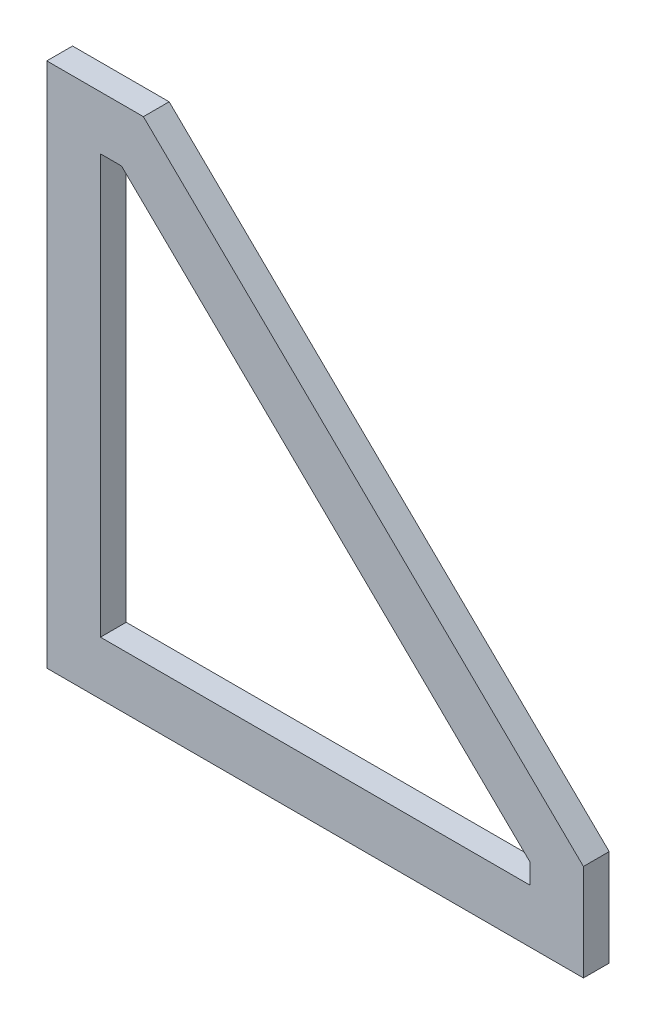
from build123d import *

# Parameters (mm, degrees)
EXTRUDE_1_DEPTH = 6


with BuildPart() as part:
    # 草图1 → 凸台-拉伸1 (new, symmetric)
    with BuildSketch(Plane.XY):
        Polygon((0, 0), (-250, 0), (-250, 245), (-205, 245), (0, 45), align=None)
        Polygon((-225, 220), (-215.175008729, 220), (-25, 34.463406118), (-25, 25), (-225, 25), align=None, mode=Mode.SUBTRACT)
    extrude(amount=EXTRUDE_1_DEPTH, both=True)


solid = part.part
